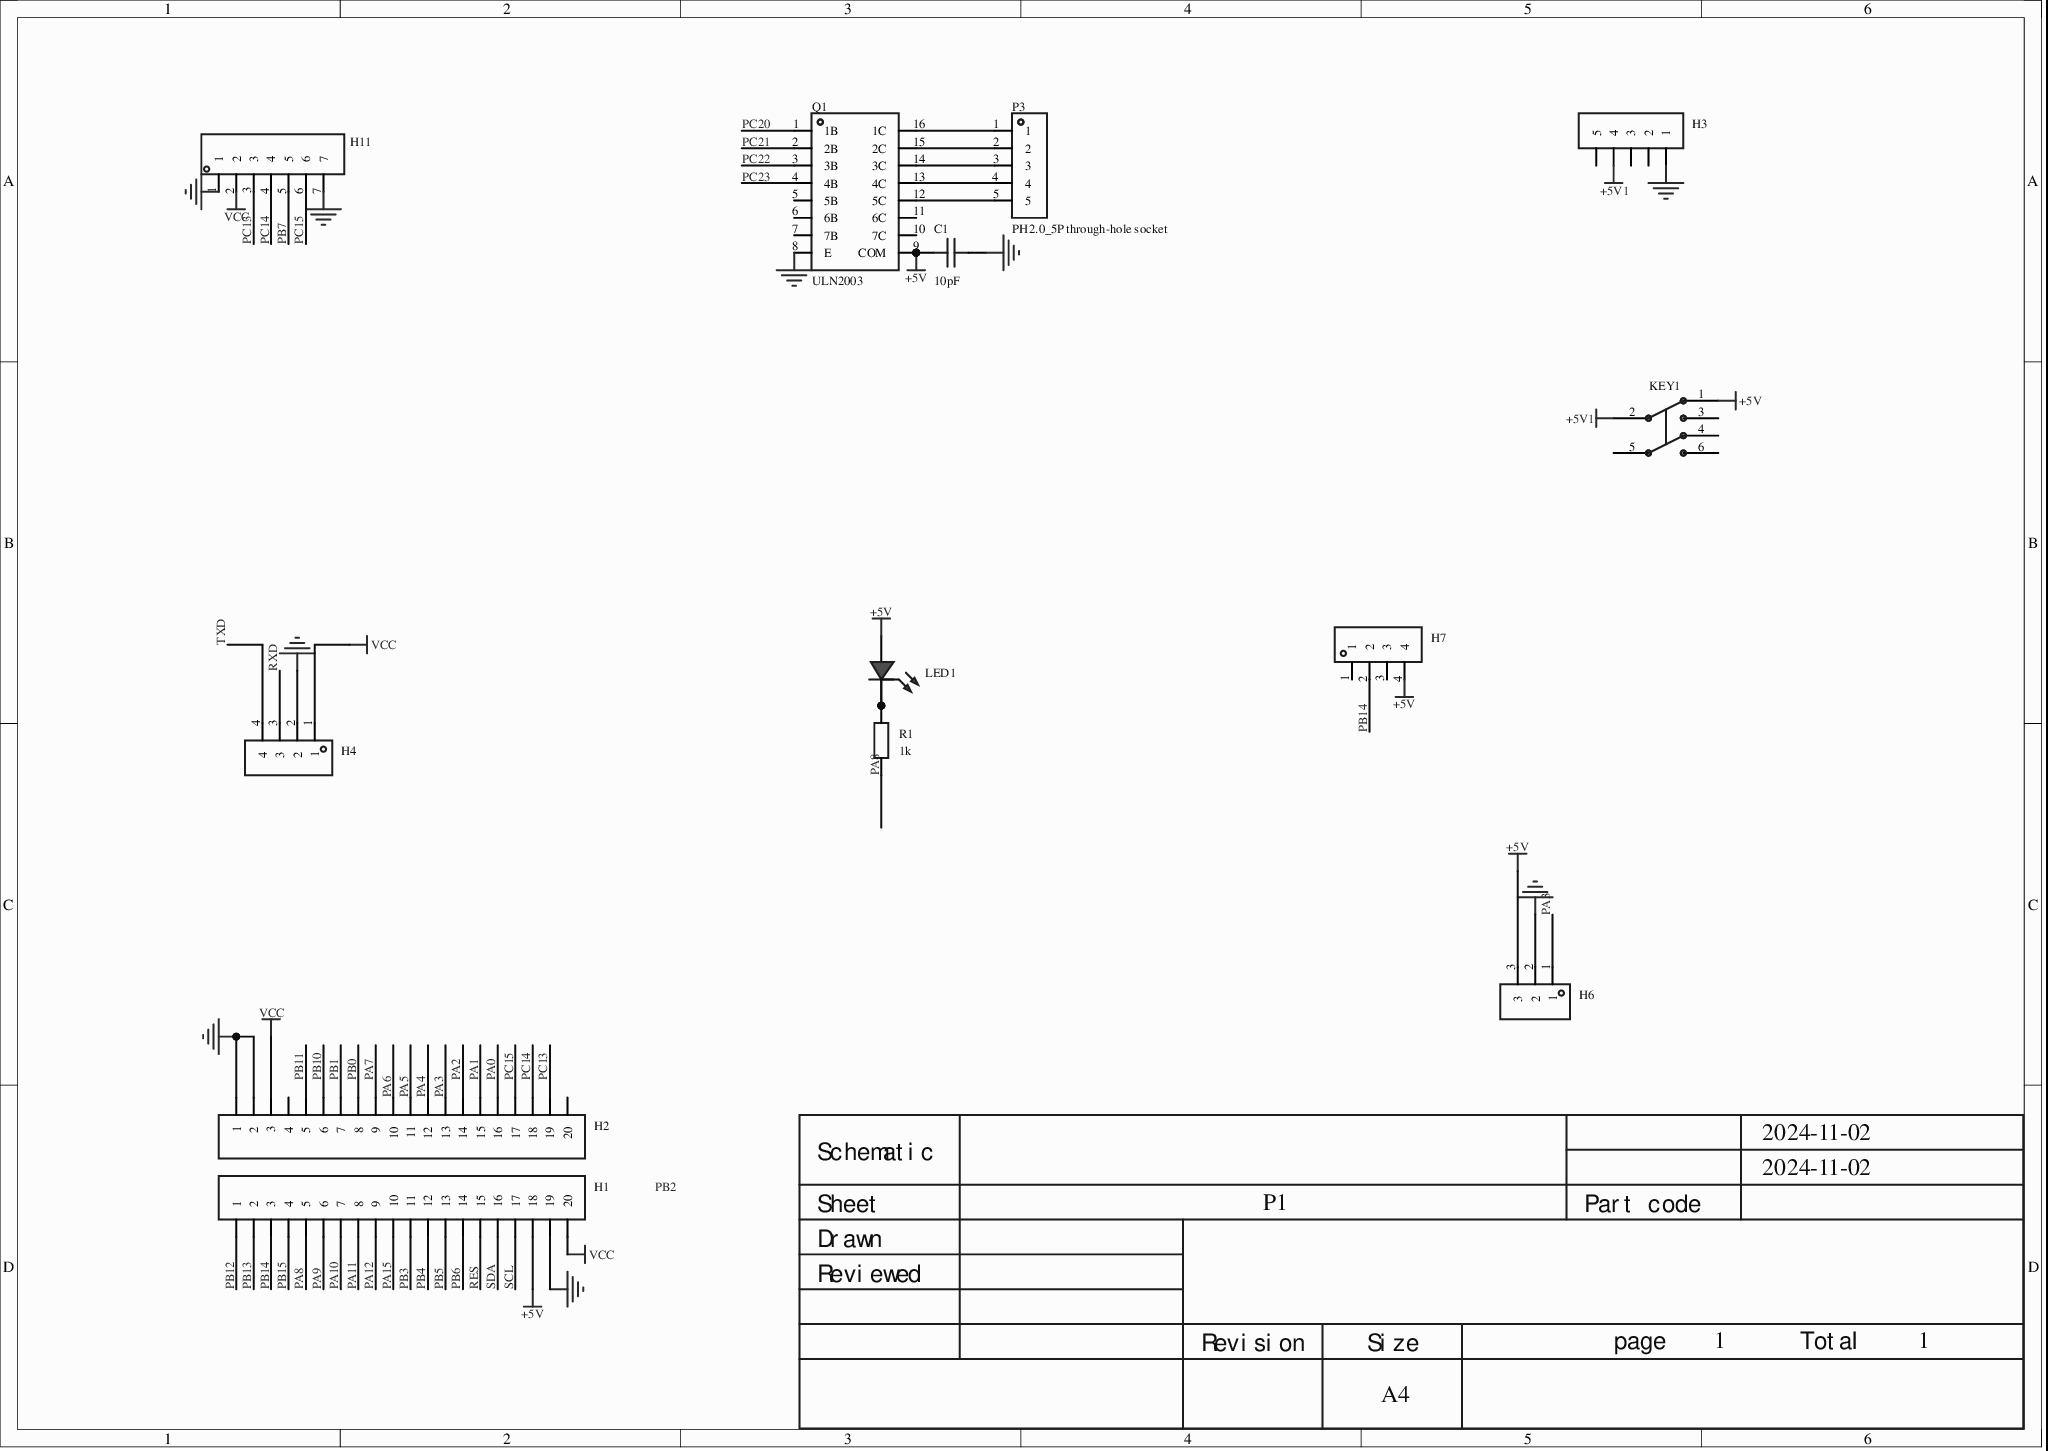
[diagram p0: MISC89064-3.schdoc]
# Altium project MISC89064-2.PrjPcb
1 sheet, 13 parts. Net scope: global (net labels, ports and power ports of the same name join across sheets).
Board file: MISC89064.pcbdoc

## Sheet MISC89064-3.schdoc
size 297 x 210 mm; Version: V1.0; @Project Name: MISC89064; @Page Count: 1; @Update Date: 2024-11-02; @Create Date: 2024-11-02; @Schematic Name: MISC89064; @Page No: 1

### Parts
C1  10pF  [CAP-TH_L5.5-W6.0-P7.50-D0.6]
H1  (no value)  [HDR-TH_20P-P2.54-V-F]
H2  (no value)  [HDR-TH_20P-P2.54-V-F]
H3  (no value)  [HDR-TH_5P-P2.54-V-F]
H4  (no value)  [HDR-TH_4P-P2.54-V-F]
H6  (no value)  [HDR-TH_3P-P2.54-V-F]
H7  (no value)  [HDR-TH_4P-P2.54-V-F]
H11  (no value)  [HDR-TH_7P-P2.54-V-F]
KEY1  Non-self-locking switch 8.5×8.5 silent  [SW-TH_6P-L8.5-W8.5-P2.54]  (value not drawn)
LED1  (no value)  [LED_TH-_5mm]
P3  PH2.0_5P through-hole socket  [CONN-TH_5P-P2.00-PH5A]
Q1  ULN2003  [DIP-16_L19.8-W6.5-P2.54-LS7.6-BL]
R1  1k  [Res_1/4W]

### Nets
+5V: C1.1 H1.18 H6.3 H7.4 KEY1.1 LED1.1(C) Q1.9(COM)
+5V1: H3.4 KEY1.2
GND: C1.2 H1.19 H2.1 H2.2 H3.1 H4.2 H6.2 H11.1 H11.7 Q1.8(E)
VCC: H1.20 H2.3 H4.1 H11.2
PA0: H2.16
PA1: H2.15
PA2: H2.14
PA3: H2.13 H6.1
PA4: H2.12
PA5: H2.11
PA6: H2.10
PA7: H2.9
PA8: H1.5 R1.1
PA9: H1.6
PA10: H1.7
PA11: H1.8
PA12: H1.9
PA15: H1.10
PB0: H2.8
PB1: H2.7
PB3: H1.11
PB4: H1.12
PB5: H1.13
PB6: H1.14
PB7: H11.5
PB10: H2.6
PB11: H2.5
PB12: H1.1
PB13: H1.2
PB14: H1.3 H7.2
PB15: H1.4
PC13: H2.19 H11.3
PC14: H2.18 H11.4
PC15: H2.17 H11.6
PC20: Q1.1(1B)
PC21: Q1.2(2B)
PC22: Q1.3(3B)
PC23: Q1.4(4B)
RES: H1.15
RXD: H4.3
SCL: H1.17
SDA: H1.16
TXD: H4.4
NetLED1_2: LED1.2(A) R1.2
NetP3_1: P3.1 Q1.16(1C)
NetP3_2: P3.2 Q1.15(2C)
NetP3_3: P3.3 Q1.14(3C)
NetP3_4: P3.4 Q1.13(4C)
NetP3_5: P3.5 Q1.12(5C)

Not connected (* = marked no-connect by the designer): H2 4 20; H3 2 3 5; H7 1 3; KEY1 3 4 5 6; Q1 5(5B) 6(6B) 7(7B) 10(7C) 11(6C)

### Notes on the sheet
- Labels drawn without touching a wire or pin: PB2
- 2024-11-02
- Schematic
- Sheet
- P1
- Part code
- Reviewed
- Drawn
- Revision
- Size
- A4
- page
- 1
- Total

### Library data of the parts
C1 = CC45SL3FD100JYGNA: 容值:10pF;精度:±5%;额定电压:3kV;温度系数:SL;; Manufacturer: TDK; AddInBom: yes; ModelId: 0ef1db373759421b9594b6107b842fed; ModelTransform: 318.897,236.22,0,0,0,0,0,0,-196.85; Tolerance: ±5%; Voltage Rated: 3kV; Temperature Coefficient: SL; φD: 5.5mm; Symbol: CC45SL3FD100JYGNA; Device: CC45SL3FD100JYGNA; Supplier: LCSC; Supplier Part: C1621830; Manufacturer Part: CC45SL3FD100JYGNA; JLCPCB Part Class: Extended library; Value: 10pF; LCSC Part Name: 10pF ±5% 3kV; Supplier Footprint: 插件,P=7.5mm; Datasheet: https://atta.szlcsc.com/upload/public/pdf/source/20210501/891ECFF90505FC7194D26A460240F667.pdf; ConvertToPcb: yes; FootprintName: CAP-TH_L5.5-W6.0-P7.50-D0.6; ModelName: CAP-TH_L5.5-W6.0-P7.50-D0.6; Lead Spacing: 7.5mm
H1 H2 = HDR-F_2.54_1x20P: ConvertToPcb: yes; ModelId: db7015f7ad9d48b8a3b1188db02e3429; ModelName: HDR-F-2.54_1x20; ModelTransform: 1999.996,100,0,0,0,0,0,0,-118.11; Symbol: HDR-F_2.54_1x20P; Device: HDR-F_2.54_1x20P; AddInBom: yes; SupplierPart: C50984; Supplier Footprint: 插件; FootprintName: HDR-TH_20P-P2.54-V-F
H3 = HDR-F_2.54_1x5P: Manufacturer: BOOMELE(博穆精密); Manufacturer Part: 2.54-1*5P母; Symbol: Header-Female-2.54_1x5; ConvertToPcb: yes; ModelId: f49cb6116a3d45e5a64915bf3e00773f; ModelTransform: 519.684,98.464,0,0,0,0,0,0,-124.016; Device: HDR-F_2.54_1x5P; Supplier: LCSC; Supplier Part: C50950; JLCPCB Part Class: Extended Part; AddInBom: yes; Supplier Footprint: 插件; FootprintName: HDR-TH_5P-P2.54-V-F; ModelName: HDR-TH_5P-P2.54-V-F
H4 H7 = HDR-F_2.54_1x4P: Manufacturer: BOOMELE(博穆精密); Manufacturer Part: 2.54-1*4P母; Symbol: 2.54-1*4P female; ConvertToPcb: yes; ModelId: 57daaad411c24bd7bd5d06edf5c4d16b; ModelName: HDR-TH_4P-P2.54-F-LI-1X4P; ModelTransform: 415.7472,98.425,0,0,0,0,0,0,-118.11; Device: HDR-F_2.54_1x4P; Supplier: LCSC; Supplier Part: C2718488; JLCPCB Part Class: Extended Part; AddInBom: yes; Supplier Footprint: 插件; FootprintName: HDR-TH_4P-P2.54-V-F
H6 = HDR-F_2.54_1x3P: Symbol: PM254V-11-03-H85; ConvertToPcb: yes; ModelId: f3b3cc5aae9641bf9e56fc160cef875b; ModelName: HDR2.54-F-LI-1X3P; ModelTransform: 299.9994,100,0,0,0,0,0,0,-118.11; Device: HDR-F_2.54_1x3P; AddInBom: yes; SupplierPart: C541850; Supplier Footprint: 插件; FootprintName: HDR-TH_3P-P2.54-V-F
H11 = HDR-F_2.54_1x7P: Manufacturer: Ckmtw(灿科盟); Manufacturer Part: B-2200S07P-A120; Symbol: 220S-1*7P H=8.5MM Ytype Gold-plated; ConvertToPcb: yes; ModelId: 4c31987253bc43b9b52c17be2a6d3f91; ModelName: HDR-TH_7P-P2.54-F-LI-1X7P; ModelTransform: 715.7466,94.488,0,0,0,0,0,0,-118.11; Device: HDR-F_2.54_1x7P; Supplier: LCSC; Supplier Part: C124418; JLCPCB Part Class: Extended Part; AddInBom: yes; Supplier Footprint: 插件; FootprintName: HDR-TH_7P-P2.54-V-F
KEY1 = 无自锁开关 8.5×8.5 无声: 6脚，8.5×8.5; Symbol: No self-locking switch 8.5×8.5 silent; AddInBom: yes; ModelId: 4c72b3966b92446eb355e1bd0fb4f880; ModelTransform: 342.519,334.645,0,180,0,0,0,0,-137.795; Device: Non-self-locking switch 8.5×8.5 silent; LCSC Part Name: 无自锁开关 8.5×8.5  无声; SupplierPart: C26228; ManufacturerPart: 无自锁开关 8.5×8.5 无声; Supplier Footprint: 插件; JLCPCB Part Class: Extended library; Supplier: LCSC; ConvertToPcb: yes; FootprintName: SW-TH_6P-L8.5-W8.5-P2.54; ModelName: SW-TH_6P-L8.5-W8.5-P2.54
LED1 = LED_TH-R_5mm: ConvertToPcb: yes; ModelId: fe9cea1bdf7642cd8d9a5077ed0e2b58; ModelName: LED-TH_BD5.9-P2.54-RD_RED; ModelTransform: 222.16,238.98,581.81,180,0,0,-6,0,-220; Symbol: LED_TH-R; Device: LED_TH-R_5mm; AddInBom: yes; FootprintName: LED_TH-_5mm; Supplier Footprint: 插件
P3 = PH2.0_5P直插插座: AddInBom: yes; ModelId: f81bfd78b1844d1db3c889f191c18287; ModelTransform: 468.503,188.976,0,180,0,0,0,-26.575,-133.858; Symbol: PH2.0_5P through-hole socket; Device: PH2.0_5P through-hole socket; LCSC Part Name: PH2.0_5P直插插座; SupplierPart: C2932788; ManufacturerPart: PH2.0_5P直插插座; Supplier Footprint: TH-5P; JLCPCB Part Class: Extended library; Supplier: LCSC; ConvertToPcb: yes; FootprintName: CONN-TH_5P-P2.00-PH5A; ModelName: CONN-TH_5P-P2.00-PH5A
Q1 = ULN2003_C557872: 通道数:七路;; Manufacturer: YW(友旺); AddInBom: yes; ModelId: 1d8537d07c784a01867ee00a159e9dcc; ModelName: DIP-16_L20.0-W6.4-H3.5-LS7.62-P2.54; ModelTransform: 787.4,311.8104,0,0,0,0,-0.003,0.001,-118.11; number of channels: seven; Symbol: ULN2003_C557872; Device: ULN2003_C557872; LCSC Part Name: ULN2003; SupplierPart: C557872; ManufacturerPart: ULN2003; Supplier Footprint: DIP-16; JLCPCB Part Class: Extended library; Datasheet: https://atta.szlcsc.com/upload/public/pdf/source/20200527/C557873_2AFF25600AE9CE704FFBA5741FE31C9F.pdf; Supplier: LCSC; ConvertToPcb: yes; FootprintName: DIP-16_L19.8-W6.5-P2.54-LS7.6-BL; Description: seven
R1 = Res_AXIAL-1/4W: Symbol: Resistor; AddInBom: yes; ModelId: 463263665006444ab7a47bd11b0cf956; ModelName: RES-TH_BD2.4-L6.3-P10.30-D0.6; ModelTransform: 427.165,94.32816,0,0,0,0,0,0,-196.85; Value: 1k; Device: Res_AXIAL-1/4W; Supplier Footprint: 轴向引线; ConvertToPcb: yes; FootprintName: Res_1/4W